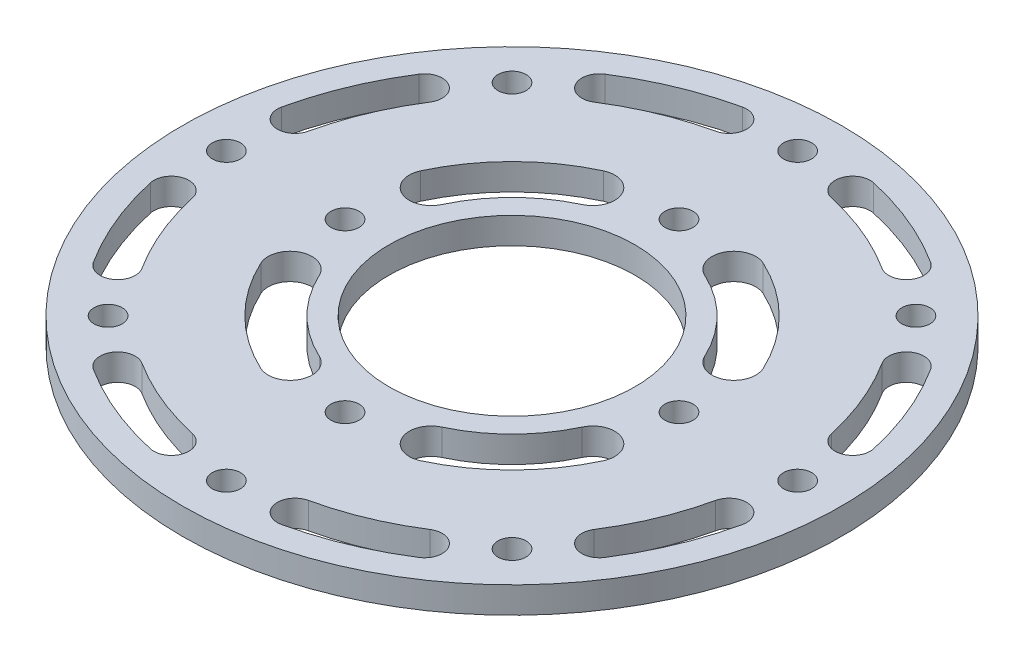
from build123d import *

# Parameters (mm, degrees)
SKETCH_1_R               = 37.5
SKETCH_1_R_2             = 1.6
SKETCH_1_R_3             = 14
EXTRUDE_1_DEPTH          = 3
CUT_EXTRUDE_1_DEPTH      = 54.117793629
CUT_EXTRUDE_1_DEPTH_BACK = 54.117793629


with BuildPart() as part:
    # 草图1 → 凸台-拉伸1 (new body)
    with BuildSketch(Plane(origin=(0, 0, 0), x_dir=(1, 0, 0), z_dir=(0, 1, 0))):
        with Locations(Location((0, 0, 0), (0, 0, 270))):
            Circle(SKETCH_1_R)
        with Locations(Location((0, 19, 0), (0, 0, 270))):
            Circle(SKETCH_1_R_2, mode=Mode.SUBTRACT)
        with Locations(Location((19, 0, 0), (0, 0, 270))):
            Circle(SKETCH_1_R_2, mode=Mode.SUBTRACT)
        with Locations(Location((0, -19, 0), (0, 0, 270))):
            Circle(SKETCH_1_R_2, mode=Mode.SUBTRACT)
        with Locations(Location((-19, 0, 0), (0, 0, 270))):
            Circle(SKETCH_1_R_2, mode=Mode.SUBTRACT)
        with Locations(Location((0, 32.5, 0), (0, 0, 270))):
            Circle(SKETCH_1_R_2, mode=Mode.SUBTRACT)
        with Locations(Location((22.980970389, 22.980970389, 0), (0, 0, 270))):
            Circle(SKETCH_1_R_2, mode=Mode.SUBTRACT)
        with Locations(Location((32.5, 0, 0), (0, 0, 270))):
            Circle(SKETCH_1_R_2, mode=Mode.SUBTRACT)
        with Locations(Location((22.980970389, -22.980970389, 0), (0, 0, 270))):
            Circle(SKETCH_1_R_2, mode=Mode.SUBTRACT)
        with Locations(Location((0, -32.5, 0), (0, 0, 270))):
            Circle(SKETCH_1_R_2, mode=Mode.SUBTRACT)
        with Locations(Location((-22.980970389, -22.980970389, 0), (0, 0, 270))):
            Circle(SKETCH_1_R_2, mode=Mode.SUBTRACT)
        with Locations(Location((-32.5, 0, 0), (0, 0, 270))):
            Circle(SKETCH_1_R_2, mode=Mode.SUBTRACT)
        with Locations(Location((-22.980970389, 22.980970389, 0), (0, 0, 270))):
            Circle(SKETCH_1_R_2, mode=Mode.SUBTRACT)
        with Locations(Location((0, 0, 0), (0, 0, 270))):
            Circle(SKETCH_1_R_3, mode=Mode.SUBTRACT)
    extrude(amount=EXTRUDE_1_DEPTH)

    # 草图2 → 切除-拉伸1 (cut, two sides: drawn at the far end of the back side and taken through both)
    with BuildSketch(Plane(origin=(0, 3, 0), x_dir=(1, 0, 0), z_dir=(0, 1, 0)).offset(-CUT_EXTRUDE_1_DEPTH_BACK)):
        with BuildLine():
            ThreePointArc((-7.467166681, 33.682212246), (-13.202578417, 31.873843872), (-18.536836488, 29.097004881))
            ThreePointArc((-18.536836488, 29.097004881), (-19.149020163, 26.335622772), (-16.387638055, 25.723439097))
            ThreePointArc((-16.387638055, 25.723439097), (-11.671844687, 28.178325742), (-6.601408225, 29.777028217))
            ThreePointArc((-6.601408225, 29.777028217), (-5.081695439, 32.162499459), (-7.467166681, 33.682212246))
        make_face()
        with BuildLine():
            ThreePointArc((-9.086292627, 19.485617421), (-15.202795796, 15.202795796), (-19.485617421, 9.086292627))
            ThreePointArc((-19.485617421, 9.086292627), (-18.276393608, 5.763977505), (-14.954078486, 6.973201319))
            ThreePointArc((-14.954078486, 6.973201319), (-11.66726189, 11.66726189), (-6.973201319, 14.954078486))
            ThreePointArc((-6.973201319, 14.954078486), (-5.763977505, 18.276393608), (-9.086292627, 19.485617421))
        make_face()
        with BuildLine():
            ThreePointArc((18.536836488, 29.097004881), (13.202578417, 31.873843872), (7.467166681, 33.682212246))
            ThreePointArc((7.467166681, 33.682212246), (5.081695439, 32.162499459), (6.601408225, 29.777028217))
            ThreePointArc((6.601408225, 29.777028217), (11.671844687, 28.178325742), (16.387638055, 25.723439097))
            ThreePointArc((16.387638055, 25.723439097), (19.149020163, 26.335622772), (18.536836488, 29.097004881))
        make_face()
        with BuildLine():
            ThreePointArc((33.682212246, 7.467166681), (31.873843872, 13.202578417), (29.097004881, 18.536836488))
            ThreePointArc((29.097004881, 18.536836488), (26.335622772, 19.149020163), (25.723439097, 16.387638055))
            ThreePointArc((25.723439097, 16.387638055), (28.178325742, 11.671844687), (29.777028217, 6.601408225))
            ThreePointArc((29.777028217, 6.601408225), (32.162499459, 5.081695439), (33.682212246, 7.467166681))
        make_face()
        with BuildLine():
            ThreePointArc((29.097004881, -18.536836488), (31.873843872, -13.202578417), (33.682212246, -7.467166681))
            ThreePointArc((33.682212246, -7.467166681), (32.162499459, -5.081695439), (29.777028217, -6.601408225))
            ThreePointArc((29.777028217, -6.601408225), (28.178325742, -11.671844687), (25.723439097, -16.387638055))
            ThreePointArc((25.723439097, -16.387638055), (26.335622772, -19.149020163), (29.097004881, -18.536836488))
        make_face()
        with BuildLine():
            ThreePointArc((7.467166681, -33.682212246), (13.202578417, -31.873843872), (18.536836488, -29.097004881))
            ThreePointArc((18.536836488, -29.097004881), (19.149020163, -26.335622772), (16.387638055, -25.723439097))
            ThreePointArc((16.387638055, -25.723439097), (11.671844687, -28.178325742), (6.601408225, -29.777028217))
            ThreePointArc((6.601408225, -29.777028217), (5.081695439, -32.162499459), (7.467166681, -33.682212246))
        make_face()
        with BuildLine():
            ThreePointArc((-18.536836488, -29.097004881), (-13.202578417, -31.873843872), (-7.467166681, -33.682212246))
            ThreePointArc((-7.467166681, -33.682212246), (-5.081695439, -32.162499459), (-6.601408225, -29.777028217))
            ThreePointArc((-6.601408225, -29.777028217), (-11.671844687, -28.178325742), (-16.387638055, -25.723439097))
            ThreePointArc((-16.387638055, -25.723439097), (-19.149020163, -26.335622772), (-18.536836488, -29.097004881))
        make_face()
        with BuildLine():
            ThreePointArc((-33.682212246, -7.467166681), (-31.873843872, -13.202578417), (-29.097004881, -18.536836488))
            ThreePointArc((-29.097004881, -18.536836488), (-26.335622772, -19.149020163), (-25.723439097, -16.387638055))
            ThreePointArc((-25.723439097, -16.387638055), (-28.178325742, -11.671844687), (-29.777028217, -6.601408225))
            ThreePointArc((-29.777028217, -6.601408225), (-32.162499459, -5.081695439), (-33.682212246, -7.467166681))
        make_face()
        with BuildLine():
            ThreePointArc((-29.097004881, 18.536836488), (-31.873843872, 13.202578417), (-33.682212246, 7.467166681))
            ThreePointArc((-33.682212246, 7.467166681), (-32.162499459, 5.081695439), (-29.777028217, 6.601408225))
            ThreePointArc((-29.777028217, 6.601408225), (-28.178325742, 11.671844687), (-25.723439097, 16.387638055))
            ThreePointArc((-25.723439097, 16.387638055), (-26.335622772, 19.149020163), (-29.097004881, 18.536836488))
        make_face()
        with BuildLine():
            ThreePointArc((19.485617421, 9.086292627), (15.202795796, 15.202795796), (9.086292627, 19.485617421))
            ThreePointArc((9.086292627, 19.485617421), (5.763977505, 18.276393608), (6.973201319, 14.954078486))
            ThreePointArc((6.973201319, 14.954078486), (11.66726189, 11.66726189), (14.954078486, 6.973201319))
            ThreePointArc((14.954078486, 6.973201319), (18.276393608, 5.763977505), (19.485617421, 9.086292627))
        make_face()
        with BuildLine():
            ThreePointArc((9.086292627, -19.485617421), (15.202795796, -15.202795796), (19.485617421, -9.086292627))
            ThreePointArc((19.485617421, -9.086292627), (18.276393608, -5.763977505), (14.954078486, -6.973201319))
            ThreePointArc((14.954078486, -6.973201319), (11.66726189, -11.66726189), (6.973201319, -14.954078486))
            ThreePointArc((6.973201319, -14.954078486), (5.763977505, -18.276393608), (9.086292627, -19.485617421))
        make_face()
        with BuildLine():
            ThreePointArc((-19.485617421, -9.086292627), (-15.202795796, -15.202795796), (-9.086292627, -19.485617421))
            ThreePointArc((-9.086292627, -19.485617421), (-5.763977505, -18.276393608), (-6.973201319, -14.954078486))
            ThreePointArc((-6.973201319, -14.954078486), (-11.66726189, -11.66726189), (-14.954078486, -6.973201319))
            ThreePointArc((-14.954078486, -6.973201319), (-18.276393608, -5.763977505), (-19.485617421, -9.086292627))
        make_face()
    extrude(amount=CUT_EXTRUDE_1_DEPTH + CUT_EXTRUDE_1_DEPTH_BACK, mode=Mode.SUBTRACT)


solid = part.part
